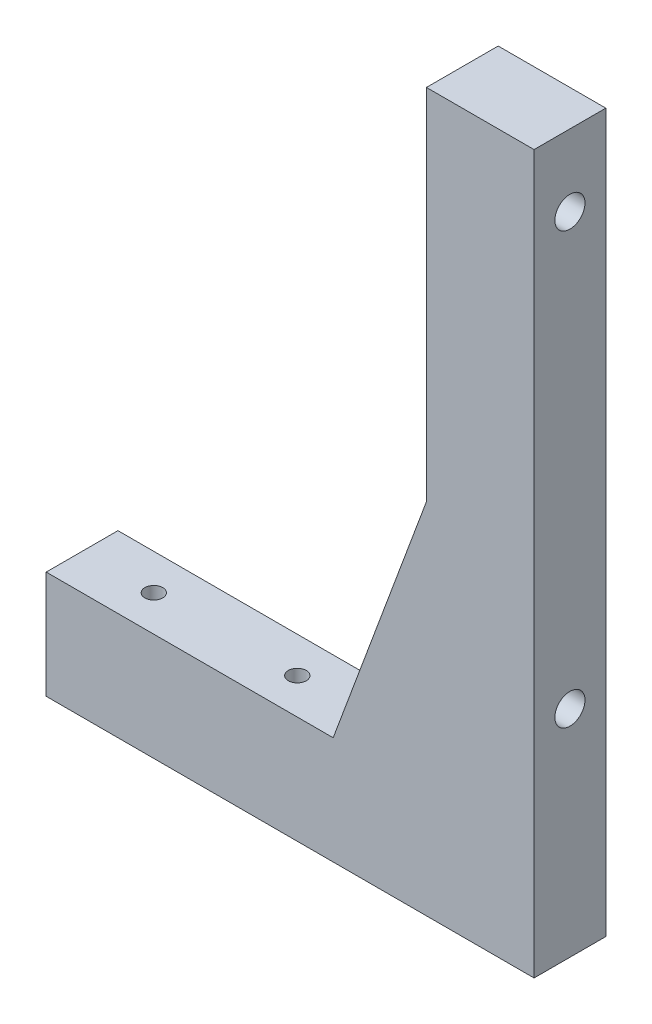
from build123d import *

# Parameters (mm, degrees)
EXTRUDE_1_DEPTH        = 5
HOLE_WIZARD_M5_1_D     = 4.2
HOLE_WIZARD_M5_1_DEPTH = 13
HOLE_WIZARD_M5_1_TIP   = 1.2618073
HOLE_WIZARD_M5_2_D     = 4.2
HOLE_WIZARD_M5_2_DEPTH = 14
HOLE_WIZARD_M5_2_TIP   = 1.2618073
HOLE_WIZARD_M3_1_D     = 2.5
HOLE_WIZARD_M3_1_DEPTH = 12.5
HOLE_WIZARD_M3_1_TIP   = 0.751075774


with BuildPart() as part:
    # 草图1 → 凸台-拉伸1 (new, symmetric)
    with BuildSketch(Plane.XY):
        Polygon((-68, 0), (-68, 15), (-28, 15), (-15, 50), (-15, 100), (0, 100), (0, 0), align=None)
    extrude(amount=EXTRUDE_1_DEPTH, both=True)

    # M5 螺纹孔1
    with Locations(Plane(origin=(0, 0, 0), x_dir=(-1, 0, 0), z_dir=(0, -1, 0))):
        with Locations((49, 0), (19, 0)):
            Hole(HOLE_WIZARD_M5_1_D / 2, depth=HOLE_WIZARD_M5_1_DEPTH)
            with Locations((0, 0, -(HOLE_WIZARD_M5_1_DEPTH + HOLE_WIZARD_M5_1_TIP / 2))):  # 118° drill point
                Cone(0, HOLE_WIZARD_M5_1_D / 2, HOLE_WIZARD_M5_1_TIP, mode=Mode.SUBTRACT)

    # M5 螺纹孔2
    with Locations(Plane(origin=(0, 0, 0), x_dir=(0, 0, -1), z_dir=(1, 0, 0))):
        with Locations((0, 30), (0, 90)):
            Hole(HOLE_WIZARD_M5_2_D / 2, depth=HOLE_WIZARD_M5_2_DEPTH)
            with Locations((0, 0, -(HOLE_WIZARD_M5_2_DEPTH + HOLE_WIZARD_M5_2_TIP / 2))):  # 118° drill point
                Cone(0, HOLE_WIZARD_M5_2_D / 2, HOLE_WIZARD_M5_2_TIP, mode=Mode.SUBTRACT)

    # M3 螺纹孔1
    with Locations(Plane(origin=(0, 15, 0), x_dir=(1, 0, 0), z_dir=(0, 1, 0))):
        with Locations((-58, 0), (-38, 0)):
            Hole(HOLE_WIZARD_M3_1_D / 2, depth=HOLE_WIZARD_M3_1_DEPTH)
            with Locations((0, 0, -(HOLE_WIZARD_M3_1_DEPTH + HOLE_WIZARD_M3_1_TIP / 2))):  # 118° drill point
                Cone(0, HOLE_WIZARD_M3_1_D / 2, HOLE_WIZARD_M3_1_TIP, mode=Mode.SUBTRACT)


solid = part.part
